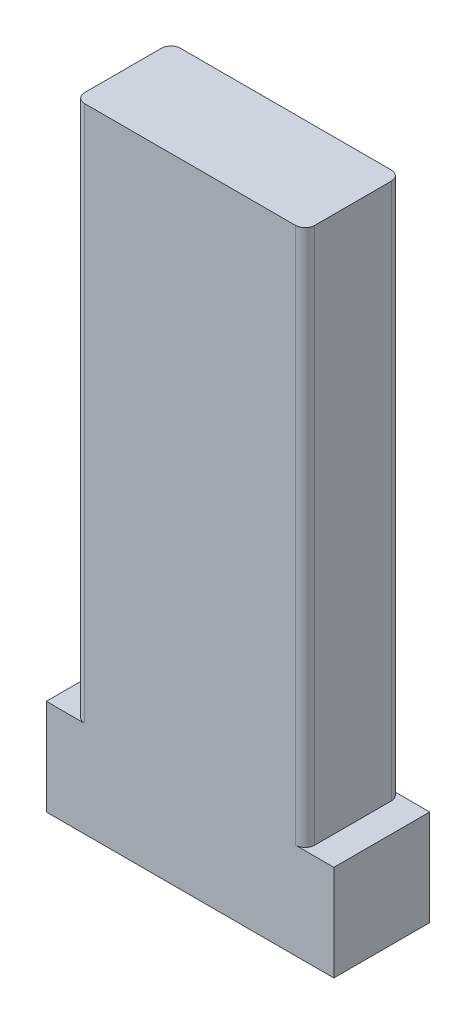
SolidWorks part; units mm, degrees
ref_plane "Front Plane" through (0, 0, 0) normal (0, 0, 1) x (1, 0, 0)
ref_plane "Top Plane" through (0, 0, 0) normal (0, 1, 0) x (1, 0, 0)
ref_plane "Right Plane" through (0, 0, 0) normal (1, 0, 0) x (0, 0, -1)
sketch "Sketch1" plane through (0, 0, 0) normal (0, 0, 1) x (1, 0, 0)
  line L0 (0, -39.77) -> (0, -52.27) construction
  line L1 (-35, -44.77) -> (35, -44.77) construction
  line L2 (7.5, -54.77) -> (-7.5, -54.77)
  line L3 (7.5, -54.77) -> (7.5, -49.77)
  line L4 (7.5, -49.77) -> (-7.5, -49.77)
  line L5 (-7.5, -54.77) -> (-7.5, -49.77)
  line L6 (7.5, -54.77) -> (-7.5, -49.77) construction
  line L7 (7.5, -49.77) -> (-7.5, -54.77) construction
  dimension "D2" = 15
  dimension "D1" = 5
  dimension "D3" = 5
extrude "Boss-Extrude1" add sketch "Sketch1" along normal mid plane 5
sketch "Sketch3" plane through (0, -49.77, 0) normal (0, 1, 0) x (1, 0, 0)
  line L1 (6, -2.5) -> (-6, -2.5)
  line L2 (6, -2.5) -> (6, 2.5)
  line L3 (6, 2.5) -> (-6, 2.5)
  line L4 (-6, -2.5) -> (-6, 2.5)
  line L5 (6, -2.5) -> (-6, 2.5) construction
  line L6 (6, 2.5) -> (-6, -2.5) construction
  point P0 (0, 0)
  dimension "D1" = 5
  dimension "D2" = 12
extrude "Boss-Extrude2" add sketch "Sketch3" along normal blind 28
fillet "Fillet1" radius 0.5 4 edges at (-6, -35.77, 2.5) (-6, -35.77, -2.5) (6, -35.77, -2.5) (6, -35.77, 2.5)
